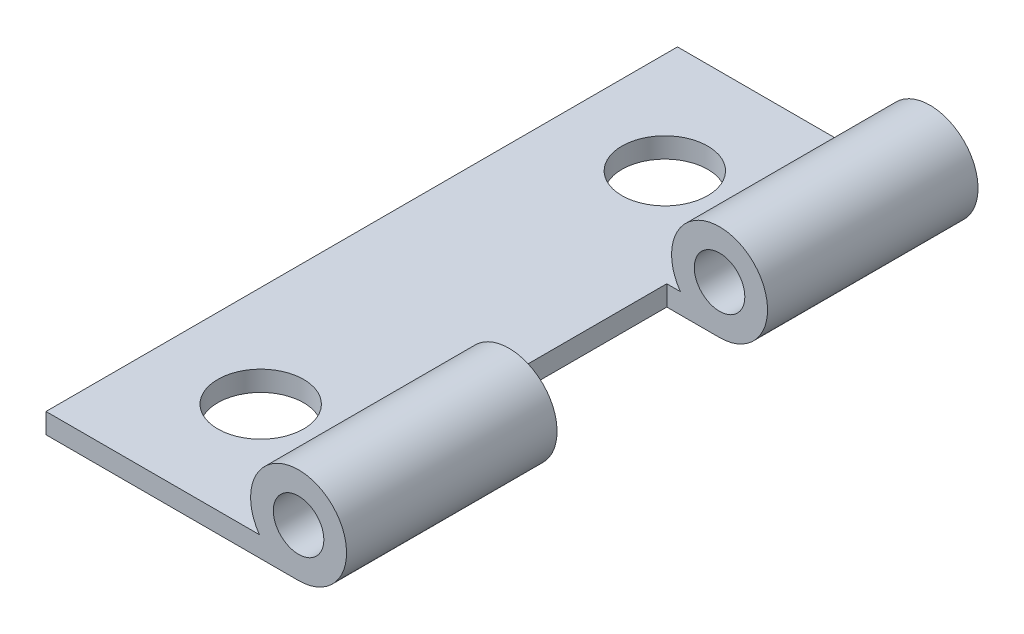
from build123d import *

# Parameters (mm, degrees)
SKETCH_1_R          = 1
EXTRUDE_1_DEPTH     = 25
CUT_EXTRUDE_1_DEPTH = 3.8
SKETCH_3_R          = 1.7
CUT_EXTRUDE_2_DEPTH = 0.8
SKETCH_4_R          = 1.7
CUT_EXTRUDE_3_DEPTH = 0.8


with BuildPart() as part:
    # 草图1 → 凸台-拉伸1 (new body)
    with BuildSketch(Plane.XY):
        with BuildLine():
            Line((-10, 0), (0, 0))
            ThreePointArc((0, 0), (0.871779789, 3.588194302), (-1.549193338, 0.8))
            Line((-1.549193338, 0.8), (-10, 0.8))
            Line((-10, 0.8), (-10, 0))
        make_face()
        with Locations((0, 1.9)):
            Circle(SKETCH_1_R, mode=Mode.SUBTRACT)
    extrude(amount=-EXTRUDE_1_DEPTH)

    # 草图2 → 切除-拉伸1 (cut)
    with BuildSketch(Plane(origin=(0, 0, 0), x_dir=(1, 0, 0), z_dir=(0, 1, 0))):
        Polygon((-2.09, 8.333333333), (2.09, 8.333333333), (2.09, 0), (6, 0), (6, 25), (2.09, 25), (2.09, 16.666666667), (-2.09, 16.666666667), align=None)
    extrude(amount=CUT_EXTRUDE_1_DEPTH, mode=Mode.SUBTRACT)

    # 草图3 → 切除-拉伸2 (cut)
    with BuildSketch(Plane(origin=(0, 0, 0), x_dir=(1, 0, 0), z_dir=(0, 1, 0))):
        with Locations(Location((-6, 20.5, 0), (0, 0, 270))):
            Circle(SKETCH_3_R)
    extrude(amount=CUT_EXTRUDE_2_DEPTH, mode=Mode.SUBTRACT)

    # 草图4 → 切除-拉伸3 (cut)
    with BuildSketch(Plane(origin=(0, 0, 0), x_dir=(1, 0, 0), z_dir=(0, 1, 0))):
        with Locations(Location((-6, 4.5, 0), (0, 0, 270))):
            Circle(SKETCH_4_R)
    extrude(amount=CUT_EXTRUDE_3_DEPTH, mode=Mode.SUBTRACT)


solid = part.part
